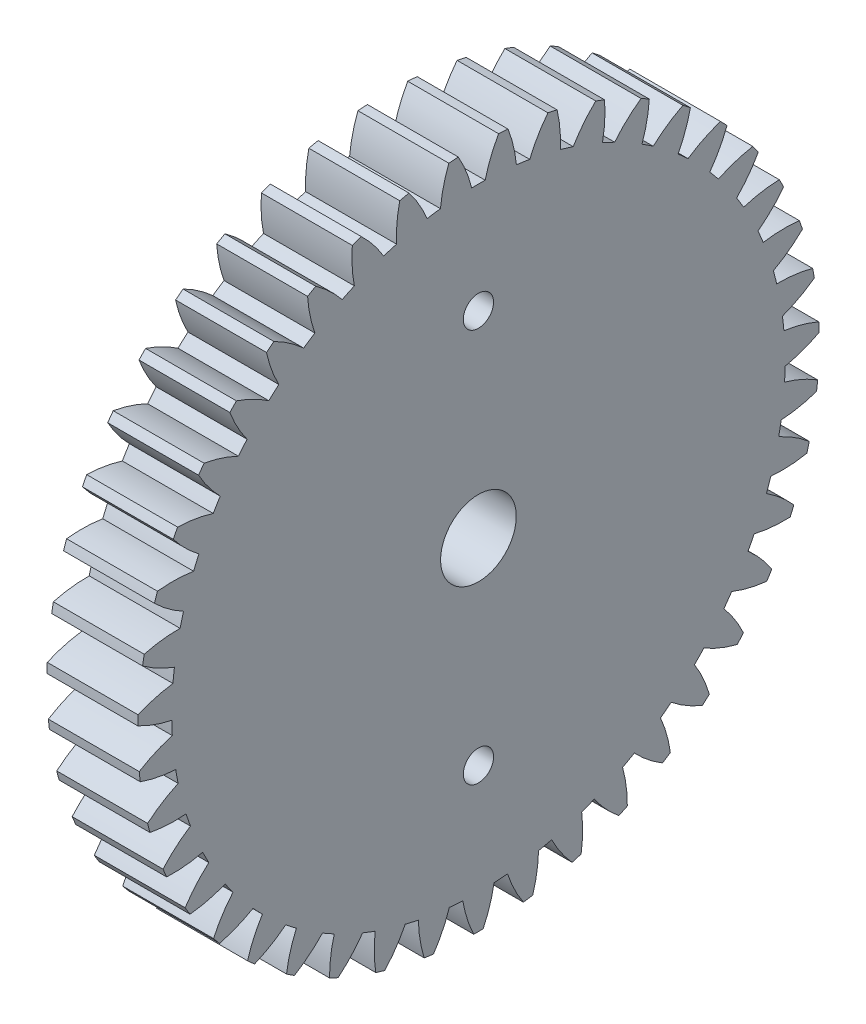
from build123d import *

# Parameters (mm, degrees)
BASPROSKE_W        = 6
BASPROSKE_H        = 22.5
TOOTHCUT_DEPTH     = 33.380549717
TEETHCUTS_COUNT    = 43
TEETHCUTS_ANGLE    = 351.627906977
BORSKE_R           = 2.5
BORE_DEPTH         = 50.0000508
SKETCH1_R          = 1
CUT_EXTRUDE1_DEPTH = 33.376524353


with BuildPart() as part:
    # BasProSke → Base-Revolve (revolve)
    with BuildSketch(Plane(origin=(0, 0, 0), x_dir=(1, 0, 0), z_dir=(0, 1, 0)), mode=Mode.PRIVATE) as base_revolve_sk:
        with Locations((3, 11.25)):
            Rectangle(BASPROSKE_W, BASPROSKE_H)
    revolve(base_revolve_sk.sketch.rotate(Axis((-10, 0, 0), (1, 0, 0)), 180), axis=Axis((-10, 0, 0), (1, 0, 0)))

    # TooCutSke → ToothCut (cut, through all)
    with BuildSketch(Plane(origin=(0, 0, 0), x_dir=(0, 0, -1), z_dir=(1, 0, 0))):
        with BuildLine():
            ThreePointArc((0.444866364, 20.244112599), (0, 20.249), (-0.444866364, 20.244112599))
            ThreePointArc((-0.444866364, 20.244112599), (-0.81630868, 21.396424265), (-1.345889069, 22.48515572))
            ThreePointArc((-1.345889069, 22.48515572), (0, 22.5254), (1.345889069, 22.48515572))
            ThreePointArc((1.345889069, 22.48515572), (0.81630868, 21.396424265), (0.444866364, 20.244112599))
        make_face()
    toothcut = extrude(amount=TOOTHCUT_DEPTH, mode=Mode.SUBTRACT)

    # TeethCuts: ToothCut ×43 about axis
    teethcuts_axis = Axis((-10, 0, 0), (1, 0, 0))
    for i in range(1, TEETHCUTS_COUNT):
        add(toothcut.rotate(teethcuts_axis, i * TEETHCUTS_ANGLE / (TEETHCUTS_COUNT - 1)), mode=Mode.SUBTRACT)

    # BorSke → Bore (cut, symmetric)
    with BuildSketch(Plane(origin=(0, 0, 0), x_dir=(0, 0, -1), z_dir=(1, 0, 0))):
        with Locations(Location((0, 0, 0), (0, 0, 180))):
            Circle(BORSKE_R)
    extrude(amount=BORE_DEPTH, both=True, mode=Mode.SUBTRACT)

    # Sketch1 → Cut-Extrude1 (cut, through all)
    with BuildSketch(Plane(origin=(6, 0, 0), x_dir=(0, 0, -1), z_dir=(1, 0, 0))):
        with Locations((0, 13)):
            Circle(SKETCH1_R)
        with Locations((0, -13)):
            Circle(SKETCH1_R)
    extrude(amount=-CUT_EXTRUDE1_DEPTH, mode=Mode.SUBTRACT)


solid = part.part
